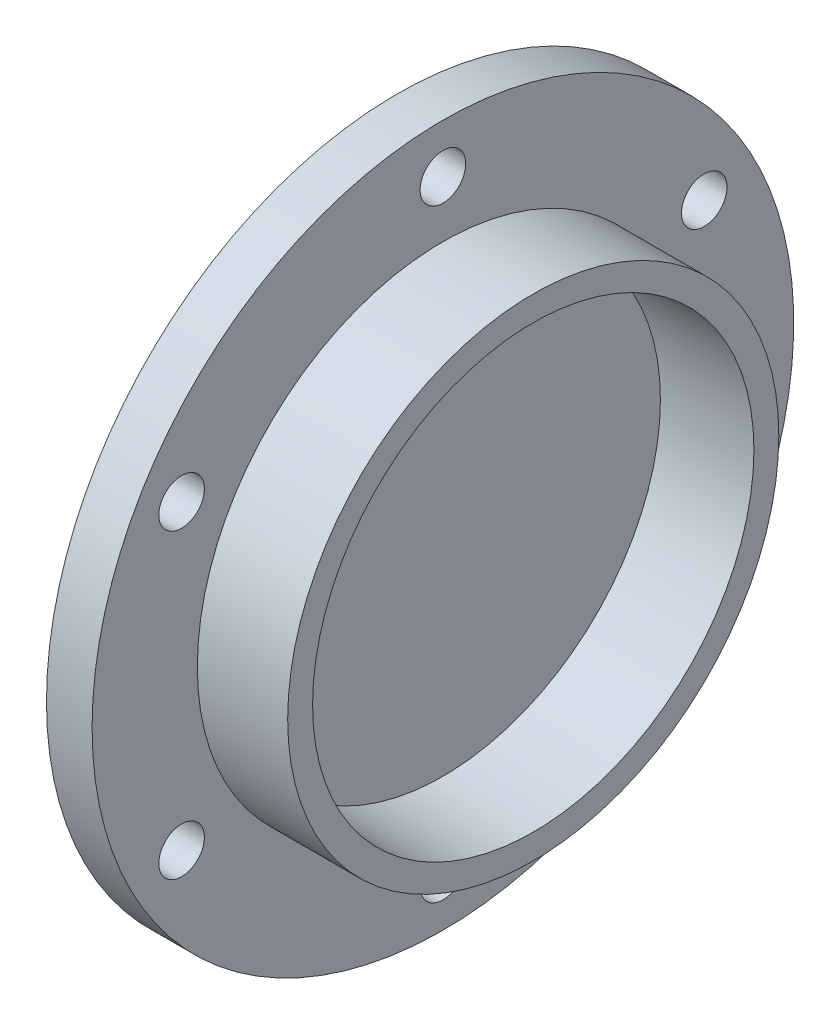
from build123d import *

# Parameters (mm, degrees)
SKETCH2_R          = 6.5
CUT_EXTRUDE2_DEPTH = 147.63411097
CIRPATTERN1_COUNT  = 6
DRAFT1_ANGLE       = 2


with BuildPart() as part:
    # Sketch1 → Revolve1 (revolve)
    with BuildSketch(Plane.XY, mode=Mode.PRIVATE) as revolve1_sk:
        Polygon((0, 0), (13, 0), (13, 62), (38.75, 62), (38.75, 70), (13, 70), (13, 100), (0, 100), align=None)
    revolve(revolve1_sk.sketch.rotate(Axis((0, 0, 0), (1, 0, 0)), 90), axis=Axis((0, 0, 0), (1, 0, 0)))

    # Sketch2 → Cut-Extrude2 (cut, through all)
    with BuildSketch(Plane.ZY):
        with Locations((0, 86)):
            Circle(SKETCH2_R)
    cut_extrude2 = extrude(amount=-CUT_EXTRUDE2_DEPTH, mode=Mode.SUBTRACT)

    # CirPattern1: Cut-Extrude2 ×6 about axis
    cirpattern1_axis = Axis((0, 0, 0), (1, 0, 0))
    for i in range(1, CIRPATTERN1_COUNT):
        add(cut_extrude2.rotate(cirpattern1_axis, i * 360 / CIRPATTERN1_COUNT), mode=Mode.SUBTRACT)

    # Draft1
    draft1_faces = [part.faces().sort_by_distance(p)[0] for p in [
        (25.875, 0, -62),
    ]]
    draft(draft1_faces, Plane(origin=(13, 0, 0), x_dir=(0, 0, 1), z_dir=(1, 0, 0)), DRAFT1_ANGLE)


solid = part.part
